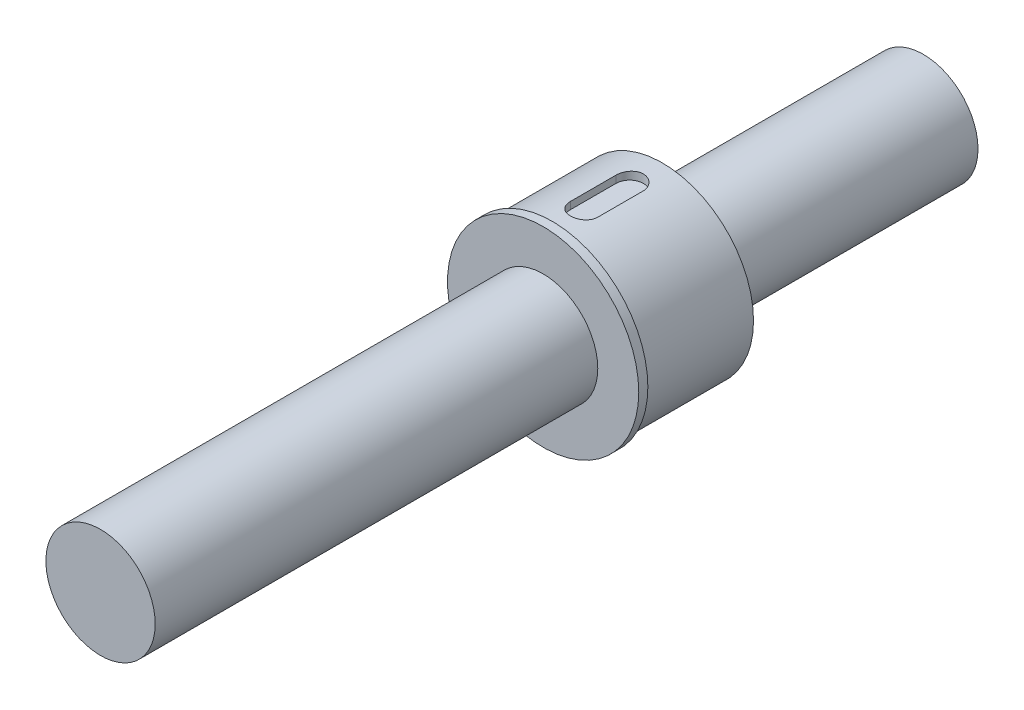
from build123d import *

# Parameters (mm, degrees)
SKETCH1_R           = 6
BOSS_EXTRUDE1_DEPTH = 28.65
SKETCH2_R           = 10
BOSS_EXTRUDE2_DEPTH = 12.1
SKETCH3_R           = 10.5
BOSS_EXTRUDE3_DEPTH = 1
SKETCH4_R           = 6
BOSS_EXTRUDE4_DEPTH = 48.6
CUT_EXTRUDE1_DEPTH  = 0.9


with BuildPart() as part:
    # Sketch1 → Boss-Extrude1 (new body)
    with BuildSketch(Plane.XY):
        Circle(SKETCH1_R)
    extrude(amount=BOSS_EXTRUDE1_DEPTH)

    # Sketch2 → Boss-Extrude2 (add)
    with BuildSketch(Plane.XY.offset(28.65)):
        Circle(SKETCH2_R)
    extrude(amount=BOSS_EXTRUDE2_DEPTH)

    # Sketch3 → Boss-Extrude3 (add)
    with BuildSketch(Plane.XY.offset(40.75)):
        Circle(SKETCH3_R)
    extrude(amount=BOSS_EXTRUDE3_DEPTH)

    # Sketch4 → Boss-Extrude4 (add)
    with BuildSketch(Plane.XY.offset(41.75)):
        Circle(SKETCH4_R)
    extrude(amount=BOSS_EXTRUDE4_DEPTH)

    # Sketch6 → Cut-Extrude1 (cut, symmetric)
    with BuildSketch(Plane(origin=(0, 10, 0), x_dir=(1, 0, 0), z_dir=(0, 1, 0))):
        with BuildLine():
            Line((1.5, -32.25), (1.5, -37.25))
            ThreePointArc((1.5, -37.25), (0, -38.75), (-1.5, -37.25))
            Line((-1.5, -37.25), (-1.5, -32.25))
            ThreePointArc((-1.5, -32.25), (0, -30.75), (1.5, -32.25))
        make_face()
    extrude(amount=CUT_EXTRUDE1_DEPTH, both=True, mode=Mode.SUBTRACT)


solid = part.part
